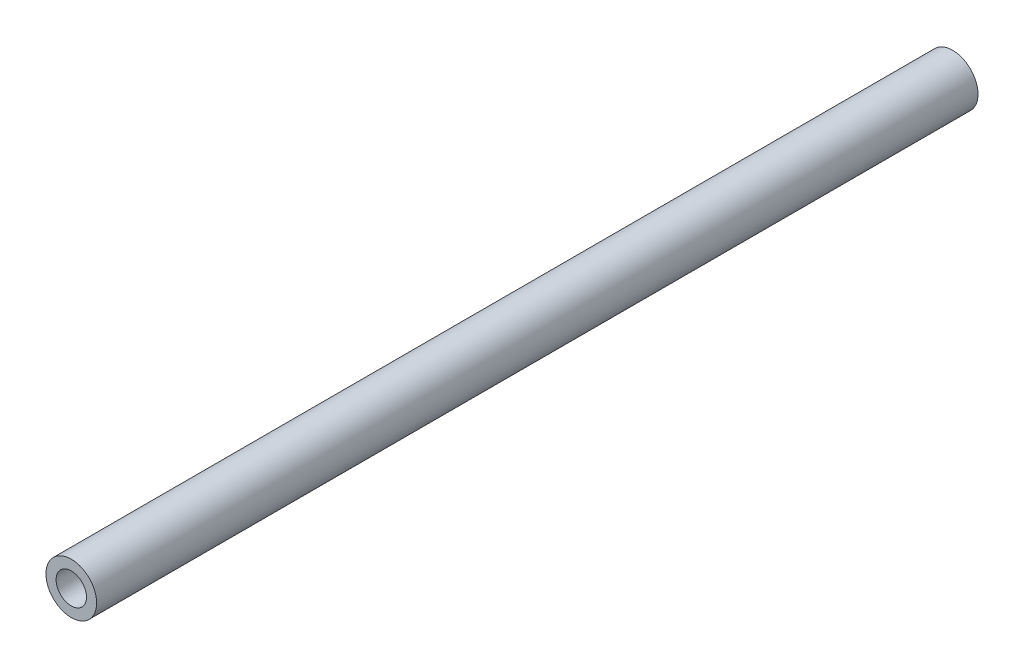
from build123d import *

# Parameters (mm, degrees)
SKETCH1_R           = 5
BOSS_EXTRUDE1_DEPTH = 87
SKETCH2_R           = 3
CUT_EXTRUDE1_DEPTH  = 10


with BuildPart() as part:
    # Sketch1 → Boss-Extrude1 (new, symmetric)
    with BuildSketch(Plane.XY):
        Circle(SKETCH1_R)
    extrude(amount=BOSS_EXTRUDE1_DEPTH, both=True)

    # Sketch2 → Cut-Extrude1 (cut)
    with BuildSketch(Plane.XY.offset(87)):
        Circle(SKETCH2_R)
    cut_extrude1 = extrude(amount=-CUT_EXTRUDE1_DEPTH, mode=Mode.SUBTRACT)

    # Mirror1: Cut-Extrude1 across plane
    add(cut_extrude1.mirror(Plane.XY), mode=Mode.SUBTRACT)


solid = part.part
